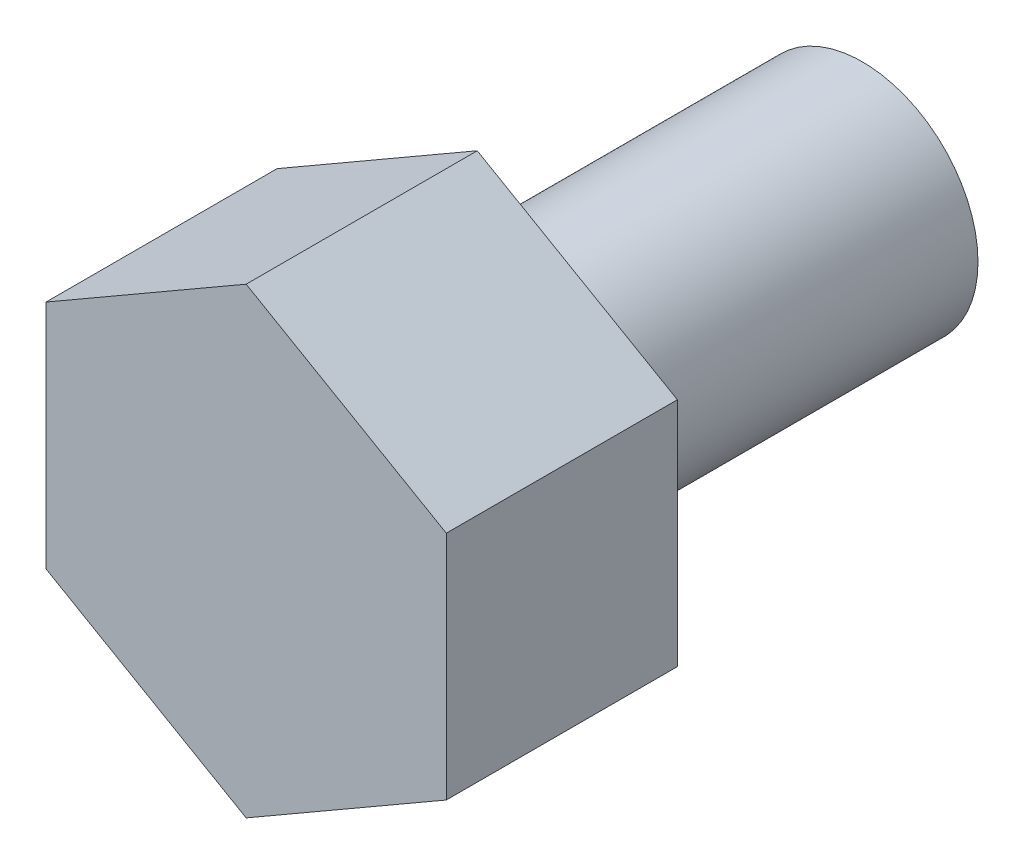
from build123d import *

# Parameters (mm, degrees)
SKETCH1_R           = 3
BOSS_EXTRUDE1_DEPTH = 10
BOSS_EXTRUDE2_DEPTH = 6


with BuildPart() as part:
    # Sketch1 → Boss-Extrude1 (new body)
    with BuildSketch(Plane.XY):
        Circle(SKETCH1_R)
    extrude(amount=BOSS_EXTRUDE1_DEPTH)

    # Sketch2 → Boss-Extrude2 (add)
    with BuildSketch(Plane.XY.offset(10)):
        Polygon((-5.196152423, -3), (0, -6), (5.196152423, -3), (5.196152423, 3), (0, 6), (-5.196152423, 3), align=None)
    extrude(amount=BOSS_EXTRUDE2_DEPTH)


solid = part.part
